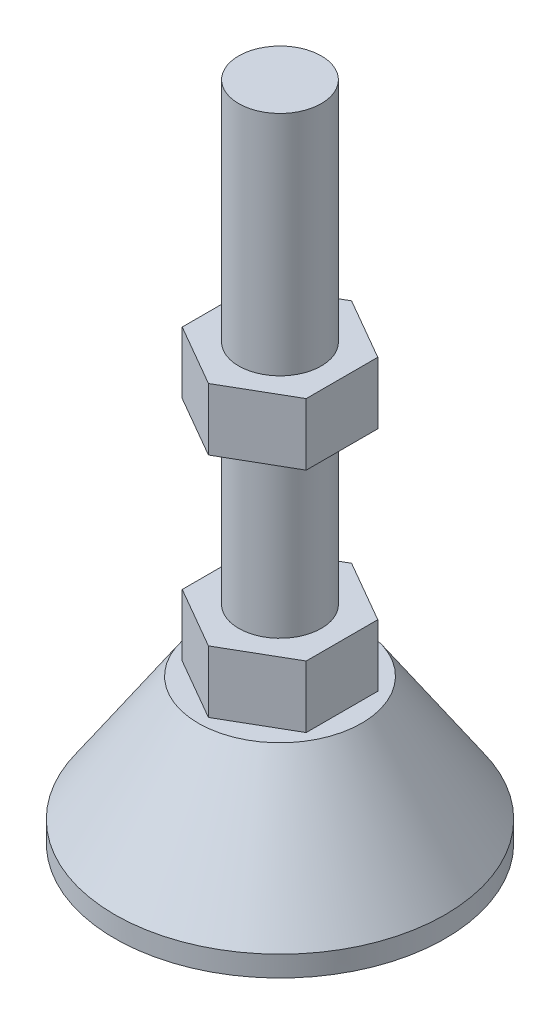
from build123d import *

# Parameters (mm, degrees)
SKETCH_1_R      = 40
EXTRUDE_1_DEPTH = 30
EXTRUDE_1_TAPER = 34
SKETCH_2_R      = 10
EXTRUDE_2_DEPTH = 125
EXTRUDE_3_DEPTH = 15
SKETCH_4_R      = 40
EXTRUDE_4_DEPTH = 5
EXTRUDE_START   = 40
EXTRUDE_5_DEPTH = 15


with BuildPart() as part:
    # 草图1 → 凸台-拉伸1 (new body)
    with BuildSketch(Plane(origin=(0, 0, 0), x_dir=(1, 0, 0), z_dir=(0, 1, 0))):
        Circle(SKETCH_1_R)
    extrude(amount=EXTRUDE_1_DEPTH, taper=EXTRUDE_1_TAPER)

    # 草图2 → 凸台-拉伸2 (add)
    with BuildSketch(Plane(origin=(0, 30, 0), x_dir=(1, 0, 0), z_dir=(0, 1, 0))):
        with Locations(Location((0, 0, 0), (0, 0, 270))):
            Circle(SKETCH_2_R)
    extrude(amount=EXTRUDE_2_DEPTH)

    # 草图3 → 凸台-拉伸3 (add)
    with BuildSketch(Plane(origin=(0, 30, 0), x_dir=(1, 0, 0), z_dir=(0, 1, 0))):
        Polygon((15, -8.660254038), (15, 8.660254038), (0, 17.320508076), (-15, 8.660254038), (-15, -8.660254038), (0, -17.320508076), align=None)
    extrude(amount=EXTRUDE_3_DEPTH)

    # 草图4 → 凸台-拉伸4 (add)
    with BuildSketch(Plane.XZ):
        with Locations(Location((0, 0, 0), (0, 0, 270))):
            Circle(SKETCH_4_R)
    extrude(amount=EXTRUDE_4_DEPTH)

    # 草图5 → 凸台-拉伸5 (add)
    with BuildSketch(Plane(origin=(0, 45, 0), x_dir=(1, 0, 0), z_dir=(0, 1, 0)).offset(EXTRUDE_START)):
        Polygon((0, -17.320508076), (15, -8.660254038), (15, 8.660254038), (0, 17.320508076), (-15, 8.660254038), (-15, -8.660254038), align=None)
    extrude(amount=EXTRUDE_5_DEPTH)


solid = part.part
